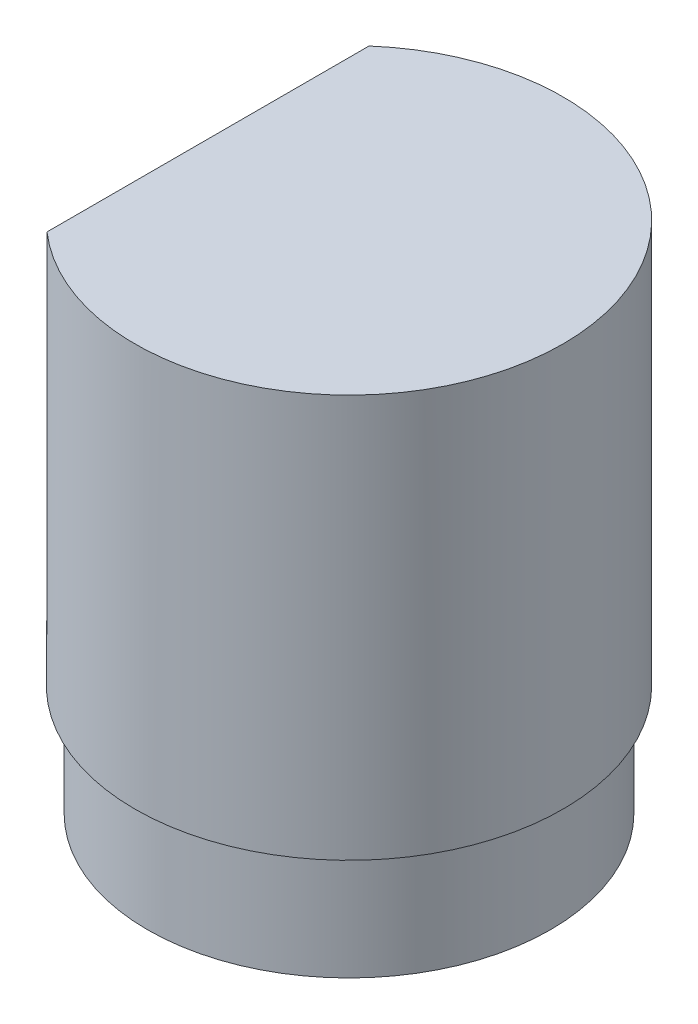
SolidWorks part; units mm, degrees
ref_plane "Front Plane" through (0, 0, 0) normal (0, 0, 1) x (1, 0, 0)
ref_plane "Top Plane" through (0, 0, 0) normal (0, 1, 0) x (1, 0, 0)
ref_plane "Right Plane" through (0, 0, 0) normal (1, 0, 0) x (0, 0, -1)
sketch "Sketch1" plane through (0, 0, 0) normal (0, 1, 0) x (1, 0, 0)
  circle A0 centre (0, 0) radius 40
  dimension "D1" = 80
extrude "Boss-Extrude1" add sketch "Sketch1" along normal blind 22
sketch "Sketch2" plane through (0, 22, 0) normal (0, 1, 0) x (1, 0, 0)
  circle A0 centre (0, 0) radius 42.5
  dimension "D1" = 85
extrude "Boss-Extrude2" add sketch "Sketch2" along normal blind 80
sketch "Sketch3" plane through (0, 0, 0) normal (1, 0, 0) x (0, 0, -1)
  line L0 (42.5, 102) -> (-42.5, 102) construction
  line L1 (-32.5, 102) -> (32.5, 102)
  line L2 (-32.5, 102) -> (-32.5, 32)
  line L3 (-32.5, 32) -> (32.5, 32)
  line L4 (32.5, 102) -> (32.5, 32)
  line L5 (-42.5, 102) -> (-42.5, 22) construction
  line L6 (42.5, 22) -> (42.5, 102) construction
  dimension "D1" = 70
  dimension "D2" = 10
  dimension "D3" = 10
extrude "Cut-Extrude1" cut sketch "Sketch3" against normal blind 80 from offset 28 offset against normal yes
sketch "Sketch4" plane through (0, 0, 0) normal (0, -1, 0) x (1, 0, 0)
  circle A0 centre (0, 0) radius 18.25
  dimension "D1" = 36.5
extrude "Cut-Extrude2" cut sketch "Sketch4" against normal blind 90
sketch "Sketch5" plane through (-28, 0, 0) normal (-1, 0, 0) x (0, 0, 1)
  line L0 (31.9726, 102) -> (-31.9726, 102) construction
  circle A0 centre (0, 72) radius 18.25
  dimension "D1" = 30
  dimension "D2" = 36.5
extrude "Cut-Extrude3" cut sketch "Sketch5" against normal blind 56
